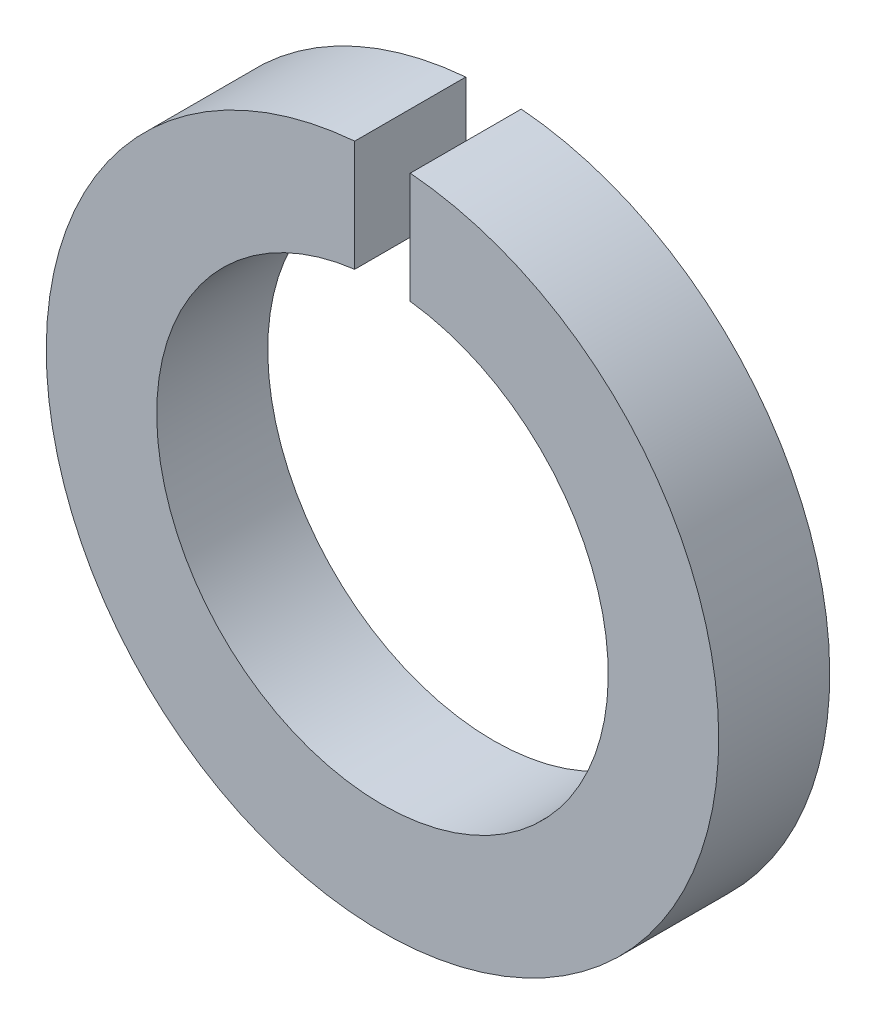
from build123d import *

# Parameters (mm, degrees)
EXTRUDE_1_DEPTH = 7.5


with BuildPart() as part:
    # 草图1 → 拉伸1 (new body)
    with BuildSketch(Plane.XY):
        with BuildLine():
            Line((-1.875, 22.634294665), (-1.875, 15.134294665))
            ThreePointArc((-1.875, 15.134294665), (0, -15.25), (1.875, 15.134294665))
            Line((1.875, 15.134294665), (1.875, 22.634294665))
            ThreePointArc((1.875, 22.634294665), (0, -22.711823352), (-1.875, 22.634294665))
        make_face()
    extrude(amount=EXTRUDE_1_DEPTH)


solid = part.part
